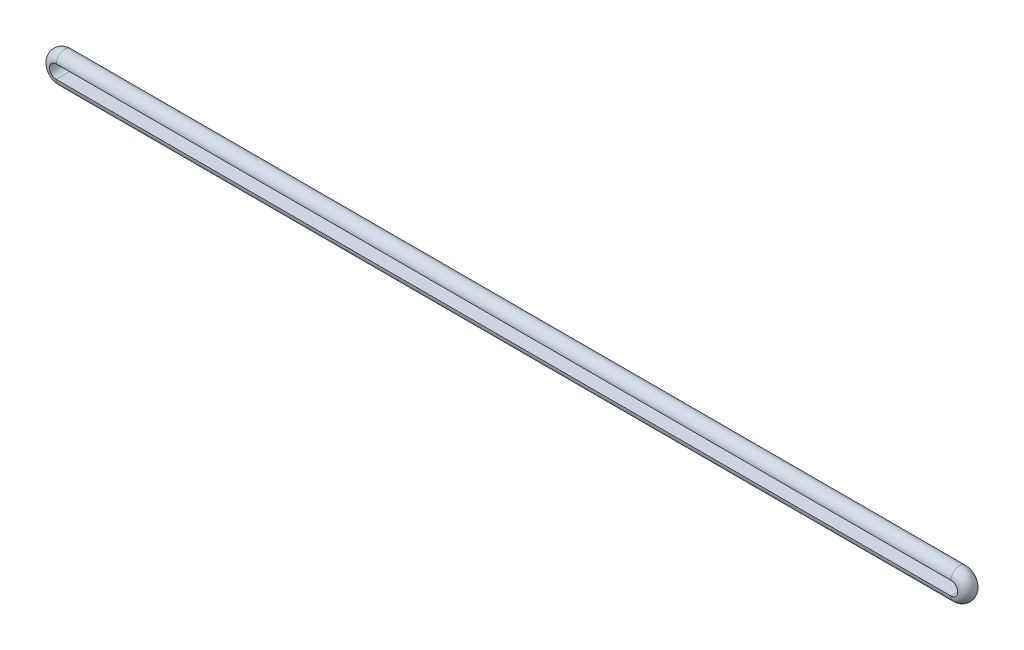
SolidWorks part; units mm, degrees
ref_plane "Front Plane" through (0, 0, 0) normal (0, 0, 1) x (1, 0, 0)
ref_plane "Top Plane" through (0, 0, 0) normal (0, 1, 0) x (1, 0, 0)
ref_plane "Right Plane" through (0, 0, 0) normal (1, 0, 0) x (0, 0, -1)
sketch "Sketch1" plane through (0, 0, 0) normal (0, 0, 1) x (1, 0, 0)
  line L0 (0, 8) -> (1060, 8)
  line L1 (0, -8) -> (1060, -8)
  arc A0 (0, 8) -> (0, -8) centre (0, 0) ccw
  arc A1 (1060, -8) -> (1060, 8) centre (1060, 0) ccw
  dimension "D1" = 1060
  dimension "D3" = 8
sketch "Sketch2" plane through (0, 0, 0) normal (1, 0, 0) x (0, 0, -1)
  line L0 (0, 8) -> (0, -8) construction
  line L1 (-10, 8) -> (10, 8)
  arc A0 (10, 8) -> (-10, 8) centre (0, 8) ccw
  dimension "D2" = 10
  dimension "D1" = 8
sweep "Sweep1" add profiles "Sketch2" path "Sketch1"
